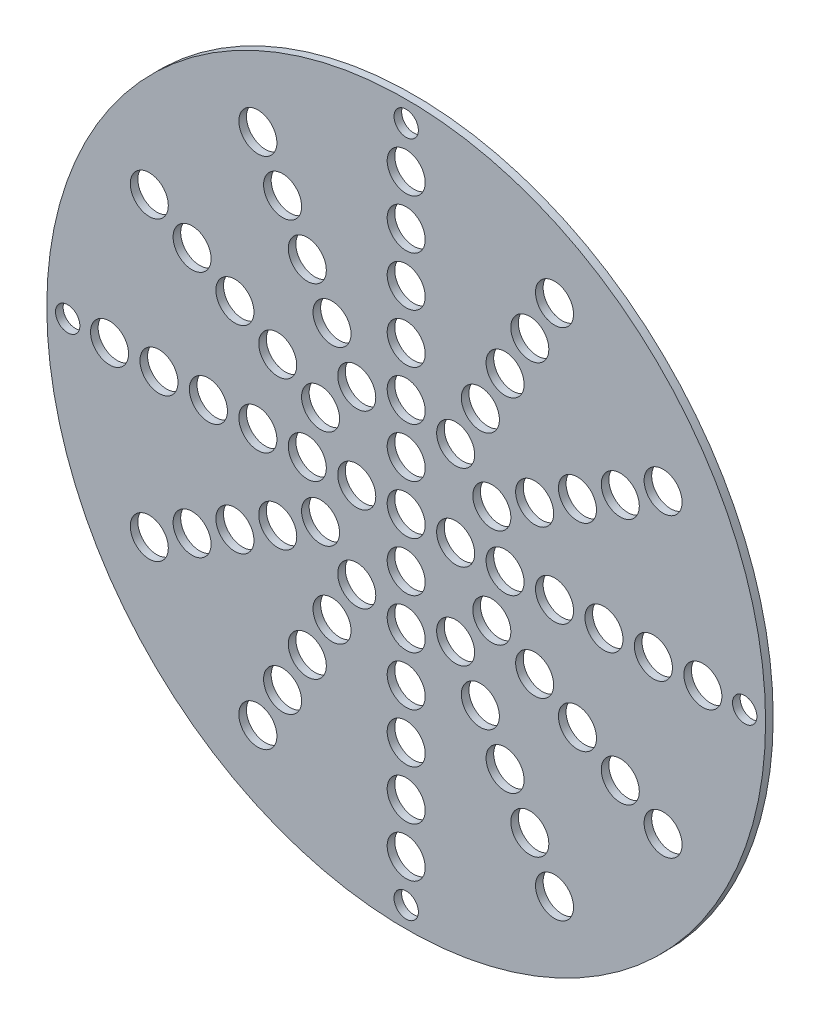
SolidWorks part; units mm, degrees
ref_plane "前视基准面" through (0, 0, 0) normal (0, 0, 1) x (1, 0, 0)
ref_plane "上视基准面" through (0, 0, 0) normal (0, 1, 0) x (1, 0, 0)
ref_plane "右视基准面" through (0, 0, 0) normal (1, 0, 0) x (0, 0, -1)
sketch "草图1" plane through (0, 0, 0) normal (0, 0, 1) x (1, 0, 0)
  circle A0 centre (0, 0) radius 47.25
  dimension "D1" = 94.5
extrude "凸台-拉伸1" add sketch "草图1" along normal blind 1
sketch "草图6" plane through (0, 0, 1) normal (0, 0, 1) x (1, 0, 0)
  line L0 (0, 0) -> (0, 29.8496) construction
  circle A0 centre (0, 6.5) radius 2.5
  circle A1 centre (0, 13) radius 2.5
  circle A2 centre (0, 19.5) radius 2.5
  circle A3 centre (0, 26) radius 2.5
  circle A4 centre (0, 32.5) radius 2.5
  circle A5 centre (0, 39) radius 2.5
  circle A110 centre (0, 0) radius 2.5
  circle A111 centre (19.5, 33.775) radius 2.5
  circle A112 centre (16.25, 28.1458) radius 2.5
  circle A113 centre (13, 22.5167) radius 2.5
  circle A114 centre (9.75, 16.8875) radius 2.5
  circle A115 centre (6.5, 11.2583) radius 2.5
  circle A116 centre (33.775, 19.5) radius 2.5
  circle A117 centre (28.1458, 16.25) radius 2.5
  circle A118 centre (22.5167, 13) radius 2.5
  circle A119 centre (16.8875, 9.75) radius 2.5
  circle A120 centre (11.2583, 6.5) radius 2.5
  circle A121 centre (39, 0) radius 2.5
  circle A122 centre (32.5, 0) radius 2.5
  circle A123 centre (26, 0) radius 2.5
  circle A124 centre (19.5, 0) radius 2.5
  circle A125 centre (13, 0) radius 2.5
  circle A126 centre (33.775, -19.5) radius 2.5
  circle A127 centre (28.1458, -16.25) radius 2.5
  circle A128 centre (22.5167, -13) radius 2.5
  circle A129 centre (16.8875, -9.75) radius 2.5
  circle A130 centre (11.2583, -6.5) radius 2.5
  circle A131 centre (19.5, -33.775) radius 2.5
  circle A132 centre (16.25, -28.1458) radius 2.5
  circle A133 centre (13, -22.5167) radius 2.5
  circle A134 centre (9.75, -16.8875) radius 2.5
  circle A135 centre (6.5, -11.2583) radius 2.5
  circle A136 centre (0, -39) radius 2.5
  circle A137 centre (0, -32.5) radius 2.5
  circle A138 centre (0, -26) radius 2.5
  circle A139 centre (0, -19.5) radius 2.5
  circle A140 centre (0, -13) radius 2.5
  circle A141 centre (-19.5, -33.775) radius 2.5
  circle A142 centre (-16.25, -28.1458) radius 2.5
  circle A143 centre (-13, -22.5167) radius 2.5
  circle A144 centre (-9.75, -16.8875) radius 2.5
  circle A145 centre (-6.5, -11.2583) radius 2.5
  circle A146 centre (-33.775, -19.5) radius 2.5
  circle A147 centre (-28.1458, -16.25) radius 2.5
  circle A148 centre (-22.5167, -13) radius 2.5
  circle A149 centre (-16.8875, -9.75) radius 2.5
  circle A150 centre (-11.2583, -6.5) radius 2.5
  circle A151 centre (-39, 0) radius 2.5
  circle A152 centre (-32.5, 0) radius 2.5
  circle A153 centre (-26, 0) radius 2.5
  circle A154 centre (-19.5, 0) radius 2.5
  circle A155 centre (-13, 0) radius 2.5
  circle A156 centre (-33.775, 19.5) radius 2.5
  circle A157 centre (-28.1458, 16.25) radius 2.5
  circle A158 centre (-22.5167, 13) radius 2.5
  circle A159 centre (-16.8875, 9.75) radius 2.5
  circle A160 centre (-11.2583, 6.5) radius 2.5
  circle A161 centre (-19.5, 33.775) radius 2.5
  circle A162 centre (-16.25, 28.1458) radius 2.5
  circle A163 centre (-13, 22.5167) radius 2.5
  circle A164 centre (-9.75, 16.8875) radius 2.5
  circle A165 centre (-6.5, 11.2583) radius 2.5
  circle A166 centre (6.5, 0) radius 2.5
  circle A167 centre (0, -6.5) radius 2.5
  circle A168 centre (-6.5, 0) radius 2.5
  point P127 (0, 0)
  point P135 (0, 0)
  dimension "D1" = 5
  dimension "D2" = 6.5
  dimension "D3" = 6.5
  dimension "D4" = 6.5
  dimension "D5" = 6.5
  dimension "D6" = 6.5
  dimension "D7" = 6.5
  dimension "D8" = 12
  dimension "D9" = 4
extrude "切除-拉伸3" cut sketch "草图6" against normal blind 2
sketch "草图7" plane through (0, 0, 1) normal (0, 0, 1) x (1, 0, 0)
  circle A0 centre (0, -44.5) radius 1.6
  circle A1 centre (44.5, 0) radius 1.6
  circle A2 centre (-44.5, 0) radius 1.6
  circle A3 centre (0, 44.5) radius 1.6
  point P12 (0, 0)
  point P13 (0, 0)
  point P14 (0, 0)
  point P15 (0, 0)
  point P16 (0, -44.4062)
  point P17 (0, -45)
  point P19 (-45, 0)
  point P21 (0, 45)
  point P23 (45, 0)
  dimension "D1" = 3.2
extrude "切除-拉伸4" cut sketch "草图7" against normal blind 2
